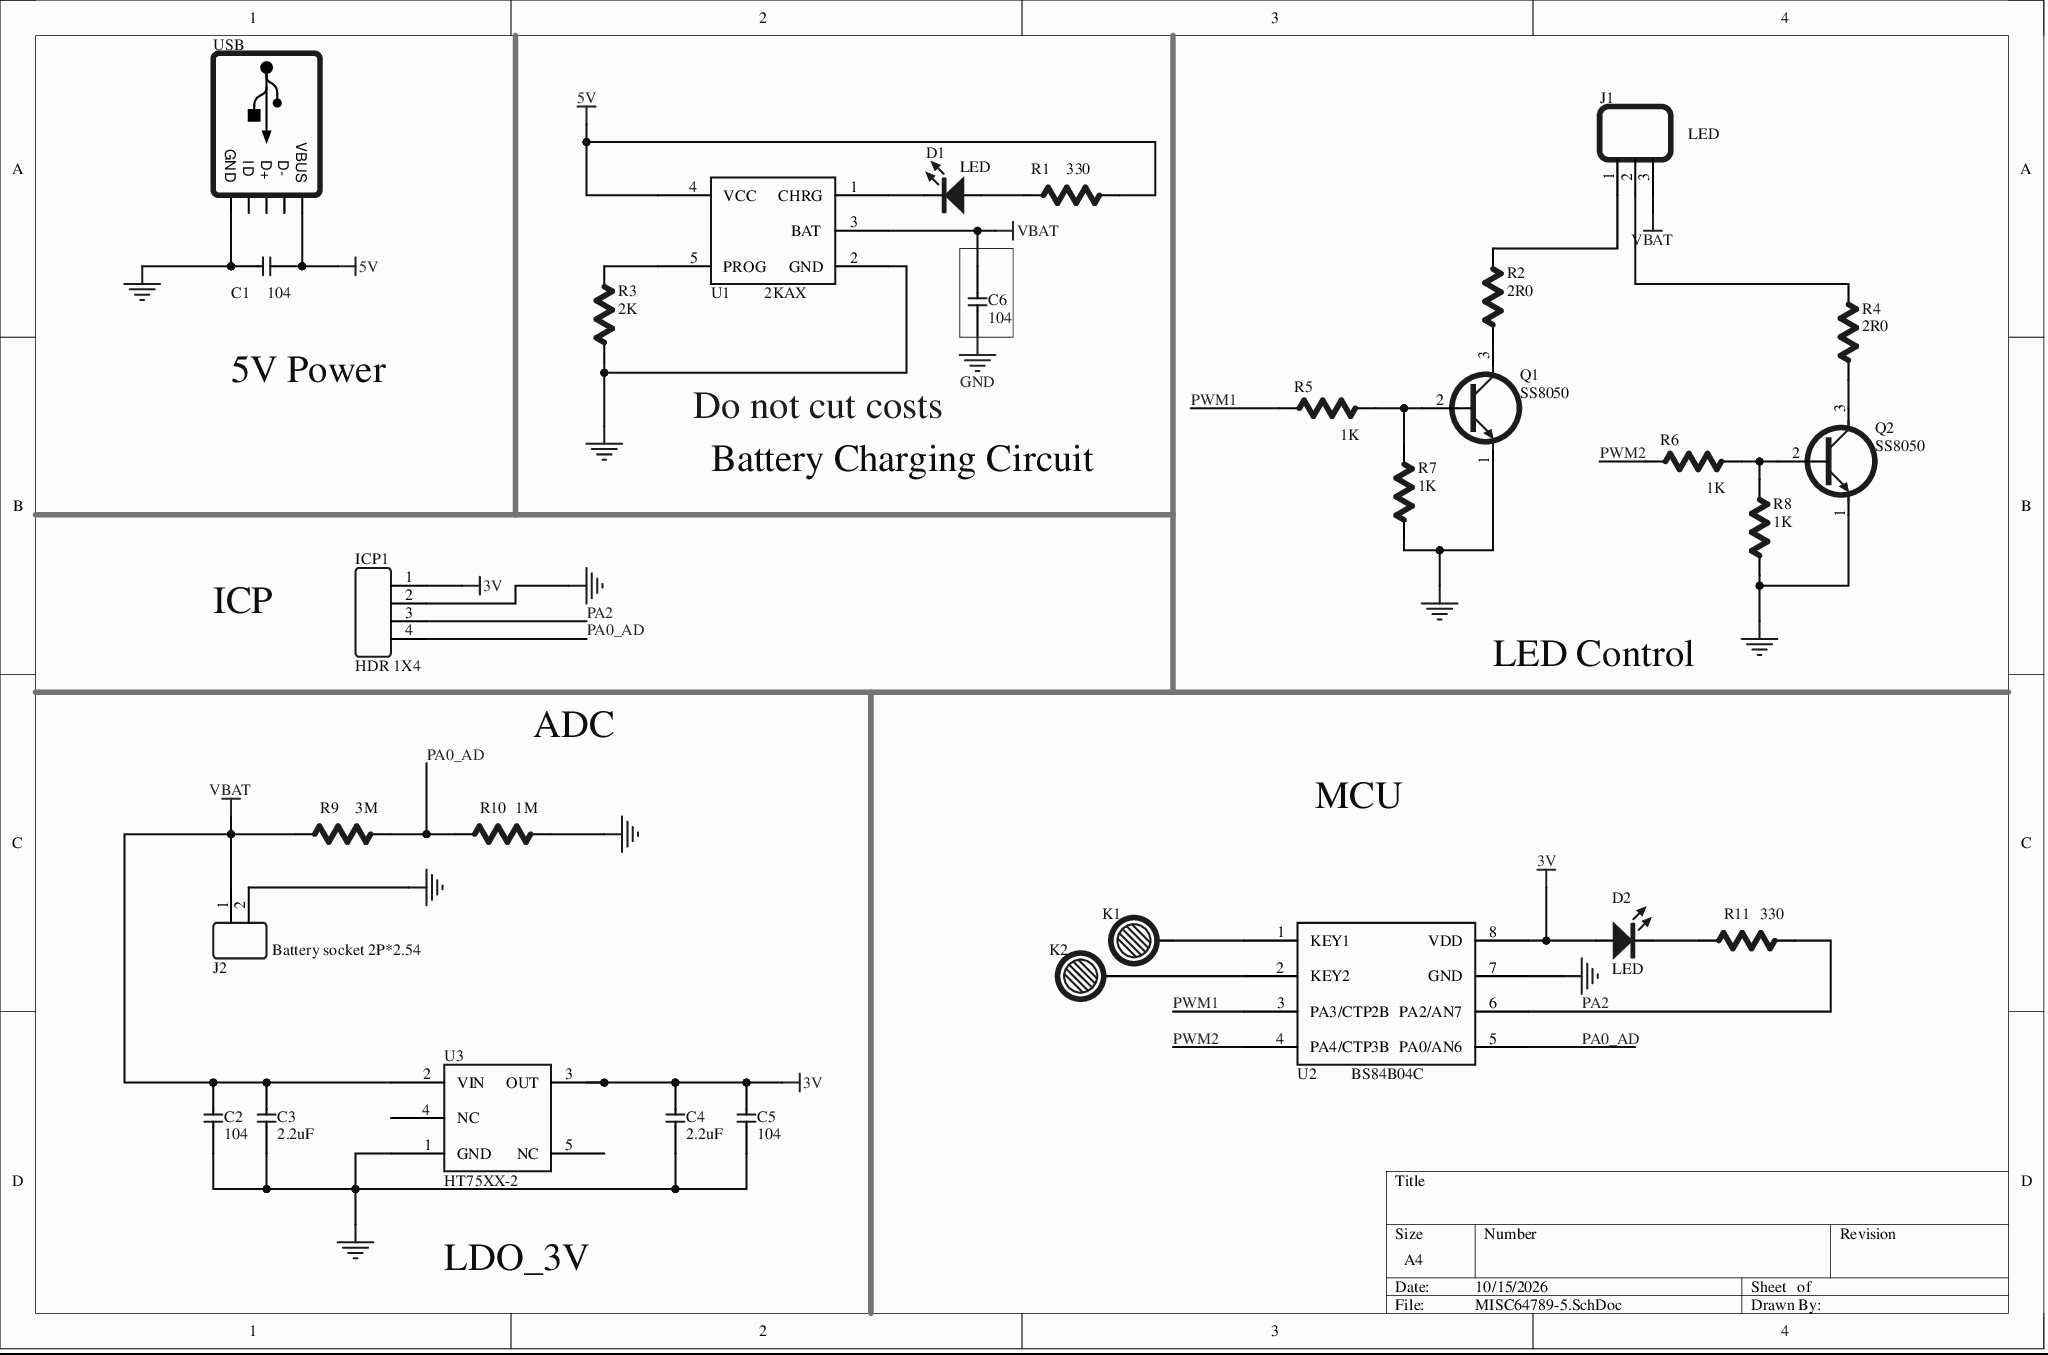
[diagram p0: MISC64789-5.SchDoc]
# Altium project MISC64789-6.PrjPcb
1 sheet, 30 parts. Net scope: global (net labels, ports and power ports of the same name join across sheets).
Board file: MISC64789.PcbDoc

## Sheet MISC64789-5.SchDoc
size A4; SheetNumber: 1; SheetTotal: 1

### Parts
C1  104  [C 0603]
C2  104  [C 0603]
C3  2.2uF  [C 0603]
C4  2.2uF  [C 0603]
C5  104  [C 0603]
C6  104  [C 0603]
D1  LED  [LED_0603]
D2  LED  [LED_0603]
ICP1  HDR 1X4  [HDR 1x4(2.54)]
J1  LED  [HDR1X3]
J2  Battery socket 2P*2.54  [HDR 1X2 Pitch 2.5mm]
K1  TOUCHKEY  [KEY]  (value not drawn)
K2  TOUCHKEY  [KEY]  (value not drawn)
Q1  SS8050  [SOT23_BJT_NPN]
Q2  SS8050  [SOT23_BJT_NPN]
R1  330  [R 0603]
R2  2R0  [R 1206]
R3  2K  [R 0603]
R4  2R0  [R 1206]
R5  1K  [R 0603]
R6  1K  [R 0603]
R7  1K  [R 0603]
R8  1K  [R 0603]
R9  3M  [R 0603]
R10  1M  [R 0603]
R11  330  [R 0603]
U1  2KAX  [SOT23 PIN-5]
U2  BS84B04C  [SOP8]
U3  HT75XX-2  [SOT23 PIN-5]
USB  USB  [Micro USB_02]  (value not drawn)

### Nets
3V: C4.2 C5.2 D2.1(A) ICP1.1 U2.8(VDD) U3.3(OUT)
5V: C1.1 R1.2 U1.4(VCC) USB.1(VDD)
GND: C1.2 C2.1 C3.1 C4.1 C5.1 C6.2 ICP1.2 J2.2 Q1.1(E) Q2.1(E) R3.1 R7.1 R8.1 R10.2 U1.2(GND) U2.7(GND) U3.1(GND) USB.5(GND)
VBAT: C2.2 C3.2 C6.1 J1.3 J2.1 R9.1 U1.3(BAT) U3.2(VIN)
PA0_AD: ICP1.4 R9.2 R10.1 U2.5(PA0/AN6)
PA2: ICP1.3 R11.2 U2.6(PA2/AN7)
PWM1: R5.1 U2.3(PA3/CTP2B)
PWM2: R6.1 U2.4(PA4/CTP3B)
NetD1_1: D1.1(A) R1.1
NetD1_2: D1.2(K) U1.1(CHRG)
NetD2_2: D2.2(K) R11.1
NetJ1_1: J1.1 R2.2
NetJ1_2: J1.2 R4.2
NetK1_1: K1.1 U2.1(KEY1)
NetK2_1: K2.1 U2.2(KEY2)
NetQ1_2: Q1.2(B) R5.2 R7.2
NetQ1_3: Q1.3(C) R2.1
NetQ2_2: Q2.2(B) R6.2 R8.2
NetQ2_3: Q2.3(C) R4.1
NetR3_2: R3.2 U1.5(PROG)

Not connected (* = marked no-connect by the designer): U3 4(NC) 5(NC); USB 2(D-) 3(D+) 4(GND)

### Notes on the sheet
- 5V Power
- Do not cut costs
- Battery Charging Circuit
- ICP
- LED Control
- ADC
- MCU
- LDO_3V

### Library data of the parts
C1 C4 C6 = Cap: ?; Layer: TOP; Footprint: C0603
  C1 C6: Value: 104
  C4: Value: 2.2uf
C2 C3 C5 = Cap: Layer: TOP; Footprint: C0603
  C2 C5: Value: 104
  C3: Value: 2.2uF
D1 D2 = LED(1): Typical INFRARED GaAs LED; Published: 8-Jun-2000; LatestRevisionDate: 08-Jul-2005; LatestRevisionNote: Mech Layer 1 removed.; PackageReference: LED-0; PackageDescription: LED; 2 Leads; Value: *; Size: Small; Update: 2016/12/29; Publisher: Altium Limited
ICP1 = HDR 1X4(?)
J1 = HDR 1X3_2
J2 = HDR 1X2(?)
K1 K2 = Touch Pad(1)
Q1 Q2 = BJT_NPN: NPN Bipolar Transistor; Published: 8-Jun-2000; LatestRevisionDate: 17-Jul-2002; LatestRevisionNote: Re-released for DXP Platform.; PackageReference: TO-226-AA; PackageDescription: TO, Flat Index; 3 In-Line, Axial Leads; Body Dia. 4.8mm; Leads 0.55 x 0.51 mm (max); Code_JEDEC: TO-226-AA; Publisher: Altium Limited
R1-R11 = Resistor(1): Resisitor; Value: *; Size: Midium; Update: 2016/12/29
U3 = HT7530
USB = USB(2_1): Mini/Micro